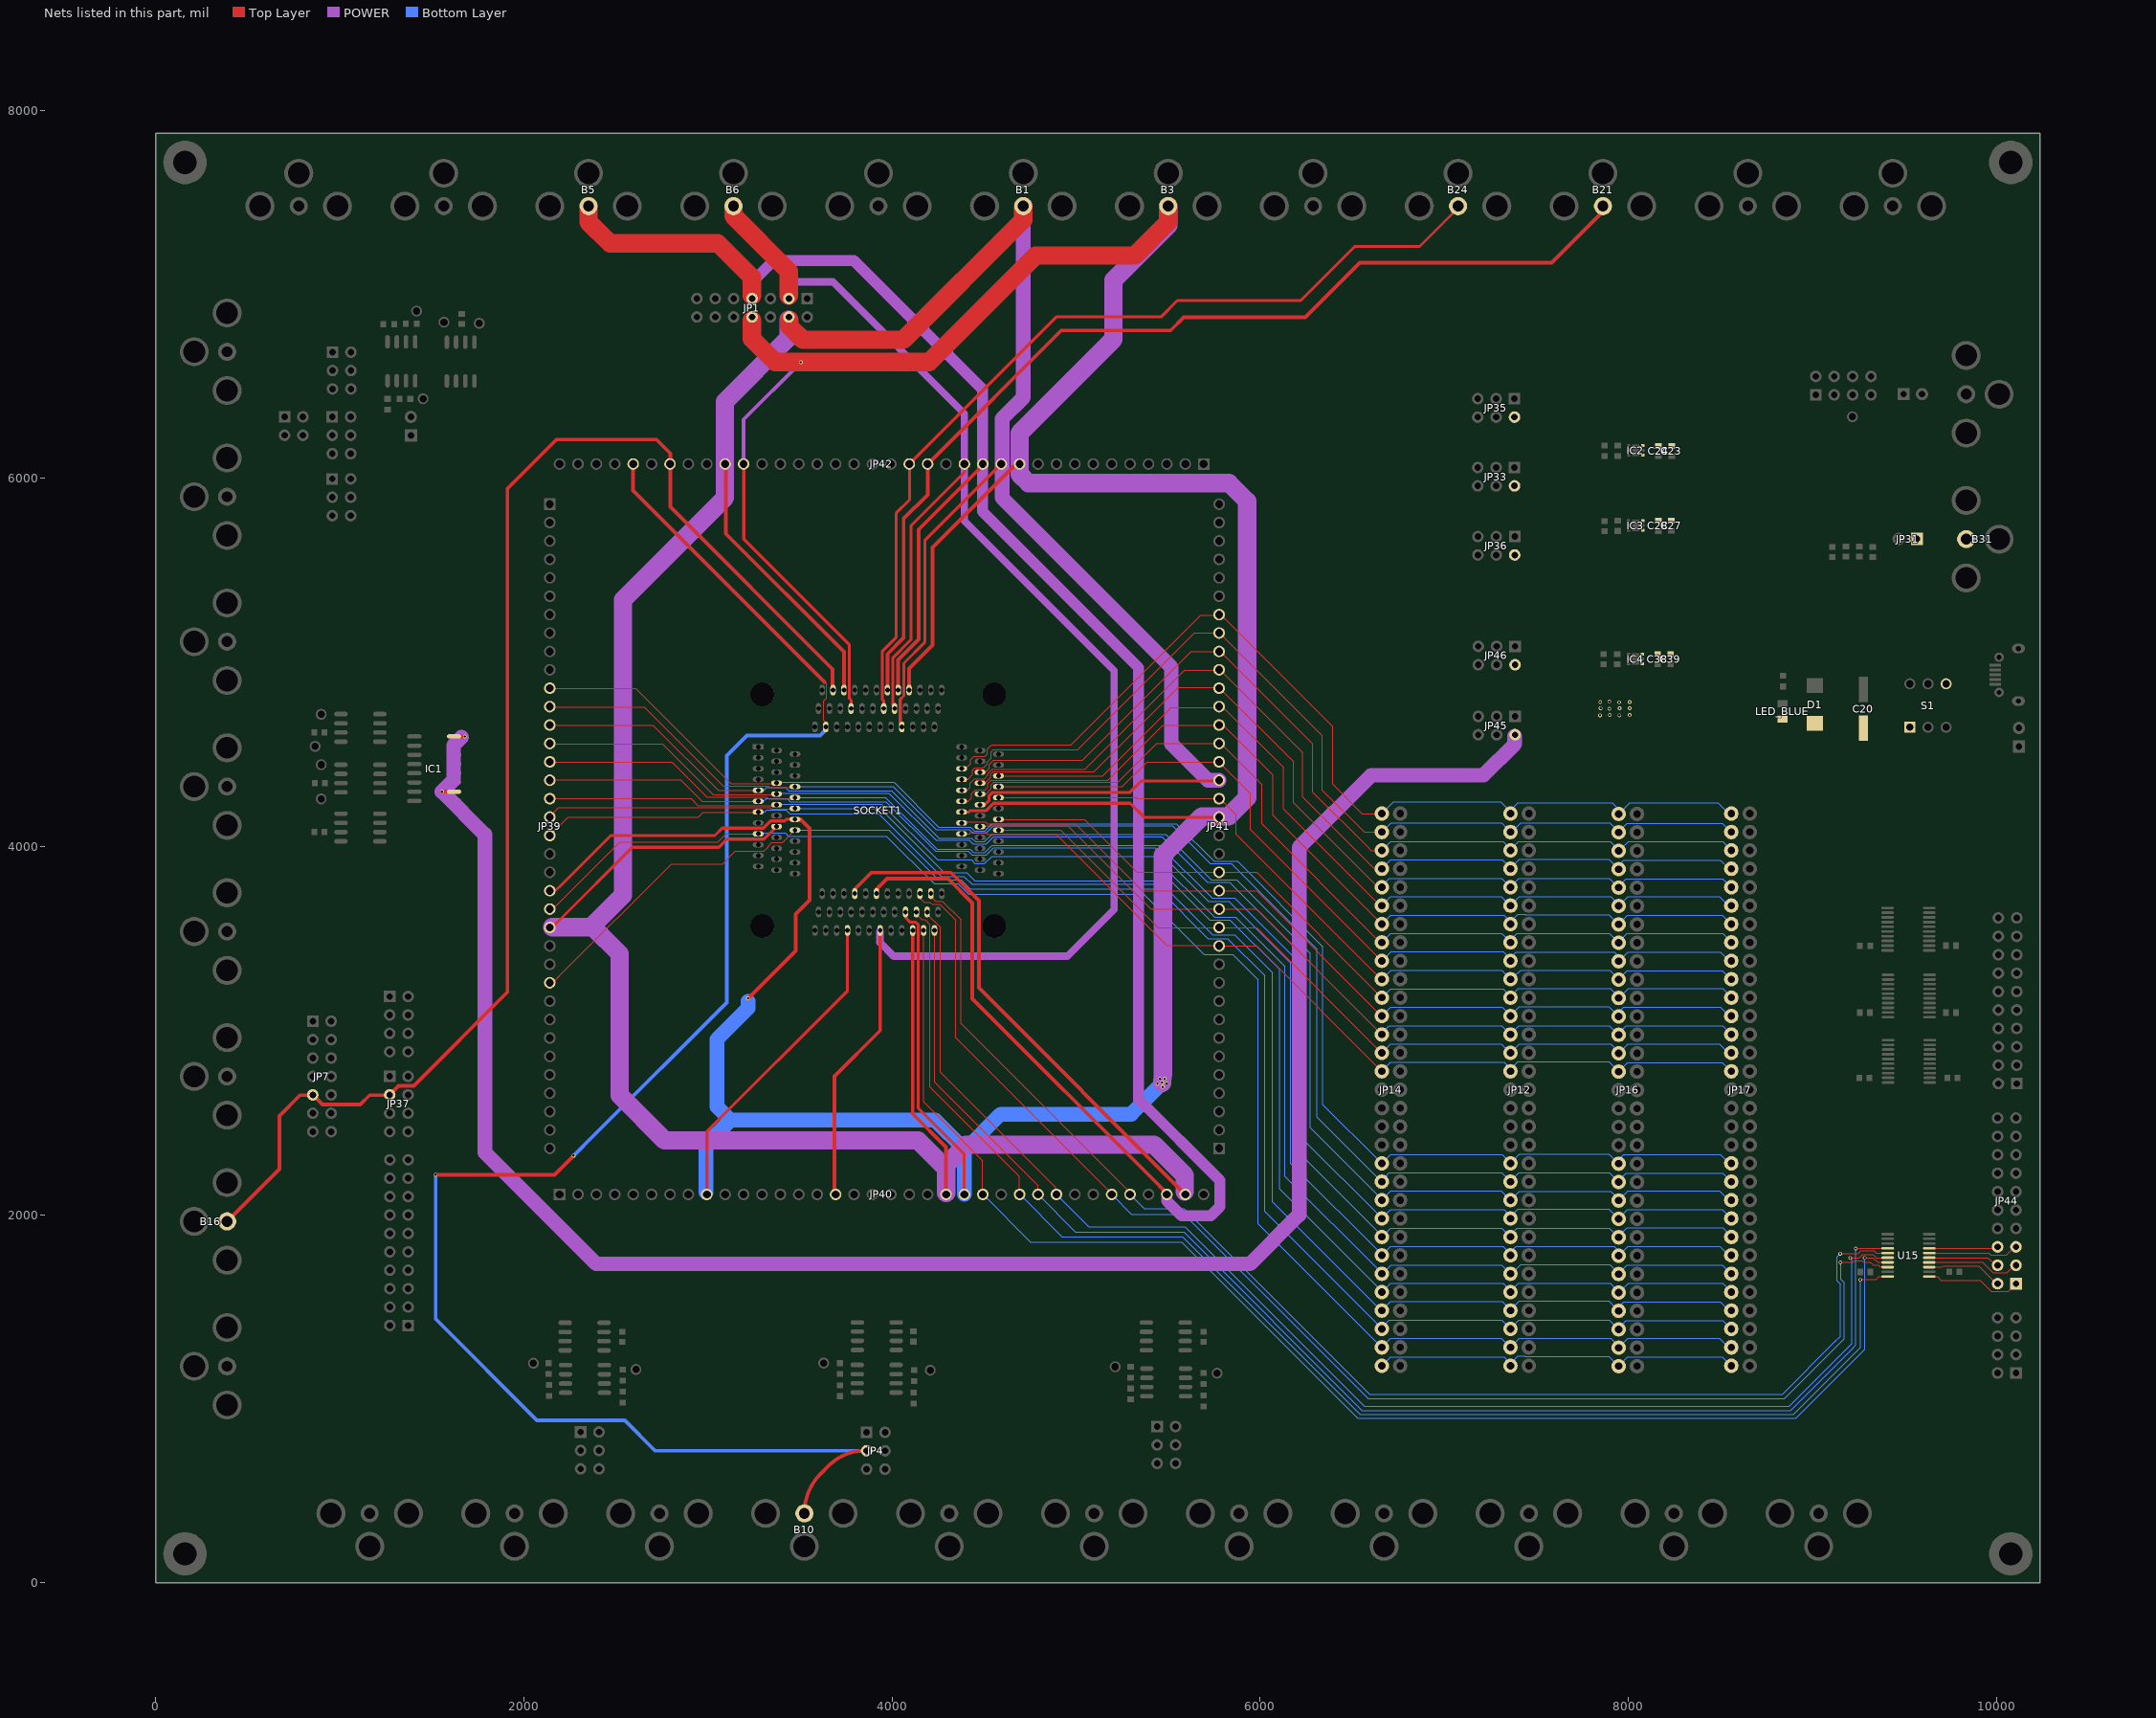
[diagram p0: the nets of this part, all layers, seen from the top]
# Altium PCB MISC62794.PcbDoc (part 5 of 7)
Units mil, origin at the board's own origin, x right, y up, seen from the top; angles counter-clockwise.
Board outline 10236.22 x 7874.02 mil, 4 copper layers (Top Layer, GND, POWER, Bottom Layer); 158 components, 185 nets, 1211 pads, 1759 vias.

## Via types
v1: diameter 20, hole 12, Top Layer to Bottom Layer, 1759 vias

## Nets (pads, with @x,y where several pads share a name; then routed paths per layer and width w, separated by ;. In a path a pad name is that pad's centre, name@x,y a point inside that pad or via, vN(x,y) a via of type N, cw(c..) or ccw(c..) an arc to the next point about the centre after c; other vN are vias at no path point) (continued)
VBIT_FORMING<4>: JP12.23 JP14.23 JP16.23 JP17.23 JP39.11 SOCKET1.11 | length 8075.9
  Top Layer w6: JP39.11@2140,4860.02 2605.98,4860.02 3125.03,4340.97 SOCKET1.11@3355.97,4340.97
  Bottom Layer w6: SOCKET1.11@3372.24,4344.65 3375.93,4348.34 4009.66,4348.34 4253.25,4104.75 4426.25,4104.75 4445.94,4085.06 4505.06,4085.06 4544.43,4124.43 5545.57,4124.43 5750.48,3919.52 5876.48,3919.52 6341,3455 6341,2598 JP14.23@6644,2295 ; JP14.23@6661,2279 6710,2328 7316,2328 7351,2293 7372,2293 7409.63,2330.63 7894.37,2330.63 7937,2288 7976,2327 8501,2327 JP17.23@8545,2283
VBIT_FORMING<5>: JP12.21 JP14.21 JP16.21 JP17.21 JP39.12 SOCKET1.12 | length 8070.4
  Top Layer w6: JP39.12@2166,4758 2654,4758 3083.03,4328.97 3327,4328.97 3334.69,4321.28 3468.56,4321.28 SOCKET1.12@3472.24,4324.97
  Bottom Layer w6: SOCKET1.12@3472.24,4324.97 4006.03,4324.97 4238.25,4092.75 4419.25,4092.75 4439,4073 4511,4073 4550.43,4112.43 5524.57,4112.43 5730,3907 5843,3907 6308,3442 6308,2530 JP14.21@6637,2201 ; JP14.21@6669,2195 6701.37,2227.37 7311.63,2227.37 JP12.21@7360,2179 ; JP12.21@7371,2192 7406.37,2227.37 7897.65,2227.37 JP16.21@7948,2177.02 ; JP16.21@7958,2196 7987.39,2225.39 8513.61,2225.39 JP17.21@8560,2179
VBIT_FORMING<6>: JP12.19 JP14.19 JP16.19 JP17.19 JP39.13 SOCKET1.13 | length 8140
  Top Layer w6: JP39.13@2140,4660.02 2700.98,4660.02 3055,4306 SOCKET1.13@3263,4306
  Bottom Layer w6: SOCKET1.13@3272.24,4305.28 3304.28,4305.28 3319,4320 3419,4320 3437.4,4301.6 3998.4,4301.6 4254.31,4045.69 4432.31,4045.69 4451.99,4026.01 4503.01,4026.01 4542.38,4065.38 5486.62,4065.38 5733,3819 5872,3819 6273,3418 6273,2472 JP14.19@6645,2100 ; JP14.19@6661,2079 6710,2128 7309,2128 JP12.19@7347,2090 ; JP12.19@7360,2079 7408.37,2127.37 7905.63,2127.37 JP16.19@7947,2086 ; JP16.19@7948,2077.02 7999.63,2128.65 8495.35,2128.65 JP17.19@8545,2079
VBIT_FORMING<7>: JP12.17 JP14.17 JP16.17 JP17.17 JP39.14 SOCKET1.14 | length 8153.6
  Top Layer w6: JP39.14@2159,4557 2752,4557 3027.09,4281.91 3368.56,4281.91 SOCKET1.14@3372.24,4285.6
  Bottom Layer w6: SOCKET1.14@3372.24,4285.6 3375.93,4289.28 3982.72,4289.28 4238.31,4033.69 4419.31,4033.69 4438.99,4014.01 4511.01,4014.01 4550.06,4053.06 5465.94,4053.06 5714,3805 5834,3805 6239,3400 6239,2402 JP14.17@6643,1998 ; JP14.17@6668,1987 6708.37,2027.37 7325.63,2027.37 7361,1992 7400,2031 7439.59,2031 7439.96,2030.63 7894.39,2030.63 JP16.17@7948,1977.02 ; JP16.17@7959,1989 7997,2027 8512,2027 JP17.17@8560,1979
VBIT_FORMING<8>: JP12.15 JP14.15 JP16.15 JP17.15 JP39.15 SOCKET1.15 | length 8237.2
  Top Layer w6: JP39.15@2140,4460.02 2803.98,4460.02 2994.09,4269.91 3320.09,4269.91 3331,4259 3462,4259 SOCKET1.15@3464,4261
  Bottom Layer w6: SOCKET1.15@3472.24,4265.91 3964.09,4265.91 4243.36,3986.64 4423.36,3986.64 4443.05,3966.95 4504.95,3966.95 4544.32,4006.32 5451.68,4006.32 5738.48,3719.52 5862.48,3719.52 6205,3377 6205,2342 JP14.15@6658,1889 ; JP14.15@6661,1879 6709.37,1927.37 7311.63,1927.37 7354,1885 7396.37,1927.37 7897.63,1927.37 7945,1880 7993.65,1928.65 8514.35,1928.65 JP17.15@8565,1878
VBIT_FORMING<9>: JP12.13 JP14.13 JP16.13 JP17.13 JP39.16 SOCKET1.16 | length 8267.5
  Top Layer w6: JP39.16@2139,4363 2851,4363 2967.77,4246.23 SOCKET1.16@3272.24,4246.23
  Bottom Layer w6: SOCKET1.16@3272.24,4246.23 3301.23,4246.23 3315,4260 3429.95,4260 3447.41,4242.54 3967.46,4242.54 4235.36,3974.64 4414.36,3974.64 4434.05,3954.95 4510.95,3954.95 4550.01,3994.01 5426.99,3994.01 5719,3702 5831,3702 6167,3366 6167,2277 JP14.13@6669,1775 ; JP14.13@6661,1779 6710,1828 7321,1828 7356,1793 7391,1828 7924,1828 7962,1790 7999,1827 8498,1827 JP17.13@8545,1780
VBIT_FORMING<10>: JP12.11 JP14.11 JP16.11 JP17.11 JP39.17 SOCKET1.17 | length 8238.2
  Top Layer w6: JP39.17@2140,4260.02 2906.98,4260.02 2944.14,4222.86 3347.86,4222.86 SOCKET1.17@3350,4225
  Bottom Layer w6: SOCKET1.17@3372.24,4226.54 3375.93,4230.23 3943.77,4230.23 4246.42,3927.58 4430.42,3927.58 4450.1,3907.9 4502.9,3907.9 4542.27,3947.27 5420.73,3947.27 5752,3616 5866,3616 6134,3348 6134,2208 JP14.11@6643,1699 ; JP14.11@6661,1679 6664.26,1679 6712.63,1727.37 7312.63,1727.37 7342,1698 7386,1698 7417,1729 7899,1729 7941,1687 7954,1687 7992.39,1725.39 8510.61,1725.39 JP17.11@8555,1681
VBIT_FORMING<11>: JP12.9 JP14.9 JP16.9 JP17.9 JP39.18 SOCKET1.18 | length 8300.9
  Top Layer w6: JP39.18@2152,4176 2186.86,4210.86 3337.14,4210.86 3344.83,4203.17 3468.56,4203.17 SOCKET1.18@3472.24,4206.86
  Bottom Layer w6: SOCKET1.18@3472.24,4206.86 3935.14,4206.86 4283,3859 4406,3859 4450,3815 5513,3815 5727.49,3600.51 5836.49,3600.51 6105,3332 6105,2140 JP14.9@6657,1588 ; JP14.9@6661,1579 6709.37,1627.37 7319.63,1627.37 7357,1590 7366,1590 7404,1628 7902,1628 7940,1590 7962,1590 8000,1628 8514,1628 JP17.9@8555,1587
VBIT_FORMING<12>: JP12.7 JP14.7 JP16.7 JP17.7 JP39.19 SOCKET1.19 | length 8380.8
  Top Layer w6: JP39.19@2140,4060.02 2240.98,4161 2947,4161 2973,4187 SOCKET1.19@3261,4187
  Bottom Layer w6: SOCKET1.19@3272.24,4187.17 3307.17,4187.17 3319,4199 3423,4199 3444,4178 3928,4178 4268,3838 4391,3838 4434,3795 5467,3795 5742.48,3519.52 5862.48,3519.52 6066,3316 6066,2070 JP14.7@6639,1497 ; JP14.7@6661,1479 6710,1528 7316,1528 7351,1493 7372,1493 7409.63,1530.63 7894.37,1530.63 7937,1488 7976,1527 8501,1527 JP17.7@8545,1483
VBIT_FORMING<13>: JP12.5 JP14.5 JP16.5 JP17.5 JP39.27 SOCKET1.24 | length 8764.5
  Top Layer w6: JP39.27@2149,3262 2158,3262 2202,3306 ; 2180,3284 2202,3306 ; SOCKET1.24@3472.24,4088.75 3404.5,4021 3346,4021 3327,4002 3327,3997.03 3304.29,3974.32 3148.32,3974.32 3080,3906 2802,3906 2202,3306
  Bottom Layer w6: SOCKET1.24@3472.24,4088.75 3883,4088.75 ; 3948.25,4088.75 3883,4088.75 ; JP14.5@6639,1404 6026,2017 6026,3298 5823.49,3500.51 5716.49,3500.51 5447,3770 4424,3770 4375,3819 4252,3819 3982.25,4088.75 3883,4088.75 ; JP14.5@6669,1395 6701.37,1427.37 7311.63,1427.37 JP12.5@7360,1379 ; JP12.5@7371,1392 7406.37,1427.37 7897.65,1427.37 JP16.5@7948,1377.02 ; JP16.5@7958,1396 7987.39,1425.39 8513.61,1425.39 JP17.5@8560,1379
VBIT_FORMING<14>: JP12.3 JP14.3 JP16.3 JP17.3 JP39.23 SOCKET1.25 | length 8606.8
  Top Layer w6: JP39.23@2149,3654 2150,3654 2521,4025 3054,4025 3098.06,4069.06 SOCKET1.25@3272.24,4069.06
  Bottom Layer w6: SOCKET1.25@3272.24,4069.06 3275.93,4072.75 SOCKET1.25@3277,4072.75 ; SOCKET1.25@3277,4069 3283,4075 3419,4075 3437,4057 3970,4057 4228,3799 4358,3799 4417,3740 5368,3740 5695,3413 5851,3413 5989,3275 5989,1951 6218,1722 JP14.3@6661,1279 6710,1328 7309,1328 JP12.3@7347,1290 ; JP12.3@7360,1279 7408.37,1327.37 7905.63,1327.37 JP16.3@7947,1286 ; JP16.3@7948,1277.02 7999.63,1328.65 8495.35,1328.65 JP17.3@8545,1279
VBIT_FORMING<15>: JP12.1 JP14.1 JP16.1 JP17.1 | length 1986.5
  Bottom Layer w6: JP14.1@6668,1187 6708.37,1227.37 7325.63,1227.37 7361,1192 7400,1231 7439.59,1231 7439.96,1230.63 7894.39,1230.63 JP16.1@7948,1177.02 ; JP16.1@7959,1189 7997,1227 8512,1227 JP17.1@8560,1179
VBIT_FORMING<16>: JP12.61 JP14.61 JP16.61 JP17.61 JP41.30 SOCKET1.102 | length 5300
  Top Layer w6: SOCKET1.102@4377.76,4423.39 4398.39,4423.39 4426,4451 4426,4473 4444,4491 4505,4491 4516.28,4502.28 4516.28,4528.28 4540,4552 4972,4552 5678,5258 JP41.30@5776,5258 ; JP41.30@5777,5260.02 5785.98,5260.02 6395,4651 6395,4338 6554,4179 JP14.61@6661,4179
  Bottom Layer w6: JP14.61@6661,4179 6724,4242 7307,4242 7356,4193 7402,4239 7913,4239 7962,4190 8009,4237 8488,4237 JP17.61@8545,4180
VBIT_FORMING<17>: JP12.57 JP14.57 JP16.57 JP17.57 JP41.28 SOCKET1.101 | length 5066.6
  Top Layer w6: SOCKET1.101@4477.76,4403.71 4507.71,4403.71 4529,4425 4529,4447 4550,4468 5034,4468 5626.02,5060.02 JP41.28@5777,5060.02 5782.98,5060.02 6286,4557 6286,4296 6584,3998 ; 6587,3995 6584,3998 ; JP14.57@6661,3979 6603,3979 6584,3998
  Bottom Layer w6: JP14.57@6661,3979 6709.37,4027.37 7319.63,4027.37 7357,3990 7366,3990 7404,4028 7902,4028 7940,3990 7962,3990 8000,4028 8514,4028 JP17.57@8555,3987
VBIT_FORMING<18>: JP12.51 JP14.51 JP16.51 JP17.51 JP41.25 SOCKET1.100 | length 4859.3
  Top Layer w6: SOCKET1.100@4577.76,4384.02 5143.02,4384.02 5515,4756 5691,4756 ; 5736.5,4756 5691,4756 ; JP41.25@5777,4760.02 5794.98,4760.02 6126,4429 6126,4204 6604,3726 ; JP41.25@5778,4758 5776,4756 5691,4756 ; 6611,3719 6604,3726 ; JP14.51@6661,3679 6651,3679 6604,3726
  Bottom Layer w6: JP14.51@6661,3679 6710,3728 7309,3728 JP12.51@7347,3690 ; JP12.51@7360,3679 7408.37,3727.37 7905.63,3727.37 JP16.51@7947,3686 ; JP16.51@7948,3677.02 7999.63,3728.65 8495.35,3728.65 JP17.51@8545,3679
VBIT_FORMING<19>: JP12.59 JP14.59 JP16.59 JP17.59 JP41.29 SOCKET1.99 | length 5265.1
  Top Layer w6: SOCKET1.99@4377.76,4364.34 4412.34,4364.34 4438,4390 4438,4415 4451,4428 4496,4428 4517,4449 4517,4452.97 4518,4453.97 4518,4460 4537,4479 4537,4514 4549,4526 5009,4526 5643.02,5160.02 JP41.29@5777,5160.02 5778.98,5160.02 6338,4601 6338,4306 6565,4079 JP14.59@6661,4079
  Bottom Layer w6: JP14.59@6661,4079 6664.26,4079 6712.63,4127.37 7312.63,4127.37 7342,4098 7386,4098 7417,4129 7899,4129 7941,4087 7954,4087 7992.39,4125.39 8510.61,4125.39 JP17.59@8555,4081
VBIT_FORMING<20>: JP12.53 JP14.53 JP16.53 JP17.53 JP41.26 SOCKET1.98 | length 4968.8
  Top Layer w6: SOCKET1.98@4477.76,4344.65 4503.65,4344.65 4535,4376 4535,4393 4549.39,4407.39 5096.39,4407.39 5554,4865 JP41.26@5777,4865 ; JP41.26@5777,4860.02 5781.98,4860.02 6181,4461 6181,4238 6600,3819 ; 6608,3811 6600,3819 ; JP14.53@6661,3779 6640,3779 6600,3819
  Bottom Layer w6: JP14.53@6669,3795 6701.37,3827.37 7311.63,3827.37 JP12.53@7360,3779 ; JP12.53@7371,3792 7406.37,3827.37 7897.65,3827.37 JP16.53@7948,3777.02 ; JP16.53@7958,3796 7987.39,3825.39 8513.61,3825.39 JP17.53@8560,3779
VBIT_FORMING<21>: JP12.45 JP14.45 JP16.45 JP17.45 JP41.22 SOCKET1.97 | length 4685.2
  Top Layer w6: SOCKET1.97@4577.76,4324.97 5250.97,4324.97 5386,4460 5395,4460 JP41.22@5777,4460.02 5777,4459 5948,4288 5948,4092 JP14.45@6661,3379
  Bottom Layer w6: JP14.45@6661,3379 6711,3429 7320,3429 7356,3393 7390.37,3427.37 7924.63,3427.37 7962,3390 7997.39,3425.39 8499.61,3425.39 JP17.45@8545,3380
VBIT_FORMING<22>: JP12.55 JP14.55 JP16.55 JP17.55 JP41.27 SOCKET1.96 | length 5187
  Top Layer w6: SOCKET1.96@4377.76,4305.28 4409.28,4305.28 4424,4320 4424,4344 4448.02,4368.02 4501.02,4368.02 4521,4388 4521,4395.97 4544.42,4419.39 5048.39,4419.39 5588,4959 5683,4959 ; 5730,4959 5683,4959 ; JP41.27@5757,4959 5683,4959 ; JP41.27@5777,4960.02 5781.98,4960.02 6232,4510 6232,4268 6597,3903 ; 6605,3895 6597,3903 ; JP14.55@6661,3879 6621,3879 6597,3903
  Bottom Layer w6: JP14.55@6661,3879 6710,3928 7316,3928 7351,3893 7372,3893 7409.63,3930.63 7894.37,3930.63 7937,3888 7976,3927 8501,3927 JP17.55@8545,3883
VBIT_FORMING<23>: JP12.47 JP14.47 JP16.47 JP17.47 JP41.23 SOCKET1.95 | length 4863.9
  Top Layer w6: SOCKET1.95@4477.76,4285.6 4508.6,4285.6 4538,4315 4538,4335 4551.34,4348.34 5226.34,4348.34 5438.02,4560.02 JP41.23@5777,4560.02 5785.98,4560.02 6009,4337 6009,4123 JP14.47@6632,3500
  Bottom Layer w6: JP14.47@6661,3479 6709.37,3527.37 7311.63,3527.37 7354,3485 7396.37,3527.37 7897.63,3527.37 7945,3480 7993.65,3528.65 8514.35,3528.65 JP17.47@8565,3478
VBIT_FORMING<24>: JP12.43 JP14.43 JP16.43 JP17.43 JP41.20 SOCKET1.94 | length 4532.7
  Top Layer w6: SOCKET1.94@4577.76,4265.91 5325.09,4265.91 ; 5325,4266 5325.09,4265.91 ; JP14.43@6651,3286 6649,3286 5870,4065 5870,4172 5781.98,4260.02 JP41.20@5777,4260.02 5330.98,4260.02 5325.09,4265.91
  Bottom Layer w6: JP14.43@6661,3279 6664.26,3279 6712.63,3327.37 7312.63,3327.37 7342,3298 7386,3298 7417,3329 7899,3329 7941,3287 7954,3287 7992.39,3325.39 8510.61,3325.39 JP17.43@8555,3281
VBIT_FORMING<25>: JP12.49 JP14.49 JP16.49 JP17.49 JP41.24 SOCKET1.93 | length 5057.6
  Top Layer w6: SOCKET1.93@4377.76,4246.23 4414.23,4246.23 4432,4264 4432,4288.05 4452.92,4308.97 4505.97,4308.97 4520,4323 4520,4343 4537.34,4360.34 5173.34,4360.34 5472,4659 5703,4659 ; 5723,4659 5703,4659 ; JP41.24@5772,4659 5703,4659 ; JP41.24@5777,4660.02 5798.98,4660.02 6070,4389 6070,4170 JP14.49@6661,3579
  Bottom Layer w6: JP14.49@6668,3587 6708.37,3627.37 7325.63,3627.37 7361,3592 7400,3631 7439.59,3631 7439.96,3630.63 7894.39,3630.63 JP16.49@7948,3577.02 ; JP16.49@7959,3589 7997,3627 8512,3627 JP17.49@8560,3579
VBIT_FORMING<26>: JP12.41 JP14.41 JP16.41 JP17.41 JP41.16 SOCKET1.88 | length 4465.3
  Top Layer w6: SOCKET1.88@4577.76,4147.8 5044.2,4147.8 5332,3860 JP41.16@5764,3860 ; JP41.16@5777,3860.02 5792,3860.02 5980,3860 JP14.41@6661,3179
  Bottom Layer w6: JP14.41@6661,3179 6709.37,3227.37 7319.63,3227.37 7357,3190 7366,3190 7404,3228 7902,3228 7940,3190 7962,3190 8000,3228 8514,3228 JP17.41@8555,3187
VBIT_FORMING<27>: JP12.39 JP14.39 JP16.39 JP17.39 JP41.15 SOCKET1.87 | length 4690.1
  Top Layer w6: SOCKET1.87@4396,4128 4401,4133 4508,4133 4516.88,4124.12 4995.88,4124.12 5359.98,3760.02 5771,3760.02 5980,3760 JP14.39@6661,3079
  Bottom Layer w6: JP14.39@6661,3079 6710,3128 7316,3128 7351,3093 7372,3093 7409.63,3130.63 7894.37,3130.63 7937,3088 7976,3127 8501,3127 JP17.39@8545,3083
VBIT_FORMING<28>: JP12.37 JP14.37 JP16.37 JP17.37 JP41.14 SOCKET1.86 | length 4615.5
  Top Layer w6: SOCKET1.86@4477.76,4108.43 4481.44,4112.12 4953.88,4112.12 5406,3660 JP41.14@5768,3660 ; JP41.14@5777,3660.02 5779,3660.02 5980,3660 JP14.37@6661,2979
  Bottom Layer w6: JP14.37@6669,2995 6701.37,3027.37 7311.63,3027.37 JP12.37@7360,2979 ; JP12.37@7371,2992 7406.37,3027.37 7897.65,3027.37 JP16.37@7948,2977.02 ; JP16.37@7958,2996 7987.39,3025.39 8513.61,3025.39 JP17.37@8560,2979
VBIT_FORMING<29>: JP12.35 JP14.35 JP16.35 JP17.35 JP41.13 SOCKET1.85 | length 4557.8
  Top Layer w6: SOCKET1.85@4592,4090 4916,4090 5445.98,3560.02 JP41.13@5777,3560.02 ; JP41.13@5775,3560 5980,3560 JP14.35@6661,2879
  Bottom Layer w6: JP14.35@6661,2879 6710,2928 7309,2928 JP12.35@7347,2890 ; JP12.35@7360,2879 7408.37,2927.37 7905.63,2927.37 JP16.35@7947,2886 ; JP16.35@7948,2877.02 7999.63,2928.65 8495.35,2928.65 JP17.35@8545,2879
VBIT_FORMING<30>: JP12.33 JP14.33 JP16.33 JP17.33 JP41.12 SOCKET1.84 | length 4805.6
  Top Layer w6: SOCKET1.84@4377.76,4069.06 4420.06,4069.06 4427,4076 4507,4076 4517.94,4065.06 4890.94,4065.06 5493,3463 JP41.12@5774,3463 ; JP41.12@5777,3460.02 5795,3460.02 5980,3460 JP14.33@6661,2779
  Bottom Layer w6: JP14.33@6668,2787 6708.37,2827.37 7325.63,2827.37 7361,2792 7400,2831 7439.59,2831 7439.96,2830.63 7894.39,2830.63 JP16.33@7948,2777.02 ; JP16.33@7959,2789 7997,2827 8512,2827 JP17.33@8560,2779
VBIT_PS_CTRL: B16.1 JP7.9 JP37.3 JP42.30 SOCKET1.139 | length 7629.6
  Top Layer w20: B16.1@386.77,1963.49 670,2246.72 670,2537 782,2649 JP7.9@835,2649 ; JP7.9@852,2651 904.5,2598.5 1110.5,2598.5 1161,2649 JP37.3@1258,2649 ; JP37.3@1269.93,2651.09 1318.83,2700 1401,2700 1910,3209 1910,5811 ; 1910,5820 1910,5811 ; SOCKET1.139@3677,4865 3677,4963 2795,5845 2795,6136 2720,6211 2176,6211 1910,5945 1910,5811
VBIT_PS_OUT1: B24.1 JP42.17 SOCKET1.125 | length 4932
  Top Layer w6: JP42.17@4093,6071 JP42.17@4093,6078.02
  Top Layer w16: SOCKET1.125@3954.53,4749.77 3954.53,4791.47 3945.84,4800.16 3945.84,5059.84 4021,5135 4021,5762 4021,5810 4095,5884 JP42.17@4095,6071 ; JP42.17@4093,6078.02 4891.98,6877 5461,6877 5550,6966 6220,6966 6514,7260 6866,7260 B24.1@7061,7455
VBIT_PS_OUT2: B21.1 JP42.16 SOCKET1.124 | length 5583.8
  Top Layer w6: SOCKET1.124@3974.21,4849.77 SOCKET1.124@3974.21,4866
  Top Layer w20: SOCKET1.124@3975,4866 3975,5046 4062,5133 4062,5780 4193,5911 JP42.16@4193,6078.02 4918.98,6804 5513,6804 5585,6876 6245,6876 6541,7172 7584,7172 B21.1@7859,7447 ; B21.1@7862.44,7447 B21.1@7862.44,7479.17
VBIT_SEL<0>: JP40.26 SOCKET1.65 U15.20 | length 7493.9
  Top Layer w6: SOCKET1.65@4131.69,3644.26 4131.69,3631.31 4160,3603 4179,3603 4206.43,3575.57 4206.43,2693.57 4692,2208 JP40.26@4692,2124 ; v1@9267,1649 9347,1649 9361.85,1663.85 U15.20@9409.97,1663.85
  Bottom Layer w6: JP40.26@4693,2110.02 4923.02,1880 5578,1880 6543,915 8898,915 9261,1278 v1(9261,1646)
VBIT_SEL<0>_MCU: JP44.1 U15.1 | length 483.8
  Top Layer w6: U15.1@9636.03,1663.85 9680.15,1663.85 9700,1644 9912,1644 9971.49,1584.51 10066.51,1584.51 JP44.1@10081,1599
VBIT_SEL<1>: JP40.31 SOCKET1.66 U15.18 | length 7376.7
  Top Layer w6: SOCKET1.66@4151.38,3744.26 4151.38,3720.62 4174,3698 4206,3698 4218,3686 4261,3686 4347,3600 4347,2960 5152,2155 ; 5162,2145 5152,2155 ; JP40.31@5183,2124 5152,2155 ; v1(9153,1741) 9221,1741 9230.5,1750.5 9271.5,1750.5 9279,1743 9315,1743 9332,1726 9359,1726 9369.97,1715.03 U15.18@9409.97,1715.03
  Bottom Layer w6: JP40.31@5193,2110.02 5300.02,2003 5587,2003 6588,1002 8849,1002 9174,1327 9174,1629 9155,1648 v1@9155,1740
VBIT_SEL<1>_MCU: JP44.2 U15.3 | length 393.5
  Top Layer w6: U15.3@9636.03,1715.03 9705.03,1715.03 9711,1721 9904,1721 JP44.2@9991,1634
VBIT_SEL<2>: JP40.24 SOCKET1.67 U15.17 | length 7737.1
  Top Layer w6: SOCKET1.67@4171.06,3544.26 4171.06,2612.94 4492,2292 4492,2262 ; JP40.24@4492,2132 4492,2262 ; 4492,2152 4492,2262 ; v1(9285,1765) 9286,1766 9330,1766 9355.38,1740.62 U15.17@9409.97,1740.62
  Bottom Layer w6: JP40.24@4493,2110.02 4751.02,1852 5573,1852 6531,894 8911,894 9285,1268 9285,1762 v1@9286,1763
VBIT_SEL<2>_MCU: JP44.3 U15.4 | length 485
  Top Layer w6: U15.4@9636.03,1740.62 9925.38,1740.62 9981.49,1684.51 10057.51,1684.51 JP44.3@10086,1713
VBIT_SEL<3>: JP40.28 SOCKET1.68 U15.16 | length 7484.5
  Top Layer w6: SOCKET1.68@4190.75,3644.26 4190.75,3631.84 4262,3560.59 4262,2774 4848,2188 ; 4882,2154 4848,2188 ; JP40.28@4889,2119 4889,2147 4848,2188 ; v1@9213,1766 9254,1766 9272,1784 9331,1784 9348.78,1766.22 U15.16@9409.97,1766.22
  Bottom Layer w6: JP40.28@4893,2110.02 5069.02,1934 5591,1934 6567,958 8874,958 9215,1299 9215,1756 v1(9206,1765)
VBIT_SEL<3>_MCU: JP44.4 U15.5 | length 372.8
  Top Layer w6: U15.5@9636.03,1766.22 9954.78,1766.22 JP44.4@9993,1728
VBIT_SEL<4>: JP40.32 SOCKET1.69 U15.15 | length 7307.9
  Top Layer w6: SOCKET1.69@4210.43,3744.26 4210.43,3729.57 4237,3703 4274,3703 4374,3603 4374,3040 5240,2174 ; 5267,2147 5240,2174 ; JP40.32@5292,2122 5240,2174 ; v1@9158,1789 9250,1789 9265,1804 9336,1804 9348.19,1791.81 U15.15@9409.97,1791.81
  Bottom Layer w6: JP40.32@5293,2110.02 5370.02,2033 5586,2033 6594,1025 8838,1025 9120.5,1307.5 ; 9128.5,1315.5 9120.5,1307.5 ; v1(9152,1788) 9134,1770 9134,1640 9153,1621 9153,1340 9120.5,1307.5
VBIT_SEL<4>_MCU: JP44.5 U15.6 | length 468.1
  Top Layer w6: U15.6@9636.03,1791.81 9958.19,1791.81 9970,1780 10054,1780 JP44.5@10086,1812
VBIT_SEL<5>: JP40.27 SOCKET1.70 U15.14 | length 7442.1
  Top Layer w6: SOCKET1.70@4230.12,3544.26 4230.12,2719.88 4792,2158 JP40.27@4792,2116 ; v1@9238.6,1817.4 U15.14@9409.97,1817.4
  Bottom Layer w6: JP40.27@4793,2110.02 4997.02,1906 5585,1906 6554,937 8882,937 9217,1272 ; 9223.5,1278.5 9217,1272 ; v1(9236,1816) 9236,1291 9217,1272
VBIT_SEL<5>_MCU: JP44.6 U15.7 | length 354.4
  Top Layer w6: U15.7@9636.03,1817.4 JP44.6@9990.4,1817.4
VCC_5V: B31.1 C20.1 C23.1 C24.1 C27.1 C28.1 C38.1 C39.1 D1.1 IC1.10 IC1.16 IC2.4 IC2.6 IC3.4 IC3.6 IC4.4 IC4.6 JP31.1 JP33.2 JP35.2 JP36.2 JP45.2 JP46.2 LED_BLUE.1 S1.1 S1.6 | length 10749.2
  Top Layer w20: v1(1554.08,4298.08) IC1.10@1619.33,4298.08 ; IC1.16@1619.33,4598.08 v1(1677.92,4598.08)
  POWER w80: 1661,4594 1617,4550 1617,4361 v1(1554.08,4298.08) 1787,4065.16 1787,2338 2392,1733 5945,1733 6212,2000 6212,3996 6603,4387 7213,4387 7383,4557 JP45.2@7383,4600
  other v1: 7847,4713 7952,4713 8008,4714 7900,4715 7897,4749 7953,4751 8008,4751 7850,4752 7951,4784 7848,4785 8008,4785 7897,4787
VDD: B6.1 JP1.3 JP40.16 JP42.14 SOCKET1.55 SOCKET1.122 | length 9463.5
  Top Layer w16: SOCKET1.122@4015,4758 4004.9,4768.1 4004.9,5025.9 4102,5123 4102,5742 4393,6033 JP42.14@4393,6078.02
  Top Layer w20: JP40.16@3687,2124 3687,2185 ; 3687,2171 3687,2185 ; SOCKET1.55@3934.84,3544.26 3934.84,2999.84 3687,2752 3687,2185
  Top Layer w40: JP1.3@3439,6977 JP1.3@3439,6994
  Top Layer w100: B6.1@3138.03,7479.17 3138.03,7425.97 3439,7125 JP1.3@3439,6994
  POWER w40: JP1.3@3439,6977 3439,7024 3483,7068 3677,7068 4393,6352 JP42.14@4393,6078.02 4393,5769 5206,4956 5206,3658 4952,3404 4009,3404 3934,3479 SOCKET1.55@3934,3539
VDD25: B5.1 JP1.7 JP40.34 JP42.13 SOCKET1.54 SOCKET1.121 | length 12283.8
  Top Layer w20: SOCKET1.54@3915.16,3744.26 3915.16,3768.16 3973,3826 4304,3826 4436,3694 4436,3173 5443.5,2165.5 ; SOCKET1.121@4033.27,4849.77 4033.27,5014.27 4144,5125 4144,5722 JP42.13@4482,6060 ; 5460,2149 5443.5,2165.5 ; JP40.34@5492,2117 5443.5,2165.5
  Top Layer w100: B5.1@2350.63,7479.17 2350.63,7393.37 2467,7277 3053,7277 3238,7092 JP1.7@3238,6994
  POWER w60: JP1.7@3239,6977 3239,7065 3357,7183 3544,7183 3792,7183 4491,6484 4491,5820 5340,4971 5340,2627 5781,2186 5781,2044 5731,1994 5573,1994 5493,2074 JP40.34@5493,2110.02
VDDC: B3.1 JP1.8 JP39.22 JP40.9 JP40.23 JP41.19 JP42.11 JP42.26 SOCKET1.21 SOCKET1.46 SOCKET1.62 SOCKET1.90 SOCKET1.118 SOCKET1.134 | length 24695.1
  Top Layer w16: JP39.22@2149,3763 2174,3763 2204.5,3793.5 ; 2192,3781 2204.5,3793.5 ; JP40.9@2994,2121 2994,2192 ; 2994,2156 2994,2192 ; JP42.26@3194,6065 3194,5671 3766.36,5098.64 3766.36,4806.64 3777.36,4795.64 SOCKET1.134@3777.36,4749.77 ; SOCKET1.21@3472.24,4147.8 3423.8,4147.8 3415,4139 3340,4139 3300.75,4099.75 3076.75,4099.75 3037,4060 2471,4060 2204.5,3793.5 ; SOCKET1.46@3757.68,3544.26 3757.68,3216.68 2994,2453 2994,2192 ; SOCKET1.62@4074,3625 4074,3613 4099,3588 4128.9,3588 4142.69,3574.2 4142.69,2577.31 4392,2328 4392,2246 ; SOCKET1.90@4377.76,4187.17 4416.17,4187.17 4424.86,4195.86 4511.48,4195.86 4550.85,4235.23 5293.77,4235.23 5370,4159 5669,4159 ; JP40.23@4392,2117 4392,2246 ; 4392,2202 4392,2246 ; 5716,4159 5669,4159 ; JP41.19@5764,4159 5669,4159
  Top Layer w20: v1(3217,3176) 3218,3176 3476,3434 3476,3634 3551,3709 3551,4099 3502.2,4147.8 SOCKET1.21@3472.24,4147.8 ; SOCKET1.118@4092.32,4849.77 4092.32,4966.32 4220,5094 4220,5625 JP42.11@4678,6083
  Top Layer w80: JP1.8@3239,6860 JP1.8@3239,6869
  Top Layer w100: JP1.8@3238,6860 3238,6759 3365,6632 4201,6632 4780,7211 5319,7211 5500.24,7392.24 B3.1@5500.24,7479.17
  POWER w20: JP42.26@3193,6078.02 3193,6320 v1(3504,6631)
  POWER w80: B3.1@5500.24,7467 B3.1@5500.24,7479.17
  POWER w100: v1@5467,2716 5470,2757 ; 5471,2762 5471,3952 5683,4164 5828,4164 5929,4265 5929,5876 5830,5975 4741,5975 4693,6023 JP42.11@4693,6078.02 4693,6246 5203,6756 5203,7077 5500.24,7374.24 B3.1@5500.24,7479.17
  Bottom Layer w80: JP40.9@2988,2121 2988,2379 3122,2513 ; 3217,3160 3217,3121 3048,2952 3048,2587 3122,2513 ; JP40.23@4393,2110.02 4393,2349 4590,2546 5299,2546 v1@5471,2718 ; 4393,2354 4234,2513 3122,2513
  other v1: 5470,2694 5442,2711 5492,2712 5467,2718 5456,2738 5481,2738
VDDH: B1.1 JP1.4 JP39.24 JP40.22 JP40.35 JP41.21 JP42.12 JP42.27 SOCKET1.23 SOCKET1.48 SOCKET1.64 SOCKET1.92 SOCKET1.120 SOCKET1.136 | length 24281.4
  Top Layer w16: JP39.24@2145,3560 2152,3560 2189,3597 ; 2181,3589 2189,3597 ; SOCKET1.23@3372.24,4108.43 3303.81,4040 3102,4040 3058,3996 2588,3996 2189,3597 ; SOCKET1.120@4054,4659 4044.27,4668.73 4044.27,4799.27 4063.95,4818.95 4063.95,4995.95 4177,5109 4177,5662.02 JP42.12@4593,6078.02 ; SOCKET1.92@4477.76,4226.54 4503.54,4226.54 4527,4250 4527,4276 4545.28,4294.28 5292.28,4294.28 5353,4355 5687,4355 ; 5710,4355 5687,4355 ; JP41.21@5767,4355 5687,4355
  Top Layer w20: JP42.27@3097,6073 3097,5699 3738,5058 SOCKET1.136@3738,4869 ; SOCKET1.48@3797.05,3744.26 3797.05,3769.05 3886,3858 4320,3858 4471,3707 4471,3232.02 JP40.35@5593,2110.02 ; SOCKET1.64@4112.01,3544.26 4112.01,2547.99 4293,2367 JP40.22@4293,2110.02
  Top Layer w80: JP1.4@3439,6868 3439,6834 3441,6832
  Top Layer w100: JP1.4@3441,6860 3441,6832 3441,6827 3515,6753 4061,6753 4712.84,7404.84 B1.1@4712.84,7479.17
  POWER w80: JP40.22@4293,2110.02 JP40.22@4293,2119 ; B1.1@4712.84,7479.17 4712.84,6439.84 4597,6324 4597,5896 4946,5547 4946,5546 5517,4975 5517,4558 5714.98,4360.02 JP41.21@5777,4360.02 ; JP40.35@5585,2117 JP40.35@5585,2125
  POWER w100: JP39.24@2153,3562 2363,3562 2537,3736 2537,5340 3092,5895 3092,6418 3439,6765 JP1.4@3439,6863 ; 2374,3562 2520,3416 2520,2648 2764,2404 4140,2404 4293.5,2250.5 ; JP40.22@4294,2119 4294,2271 4403,2380 5424,2380 5590,2214 JP40.35@5590,2125
VG1: B10.1 JP4.3 JP42.32 SOCKET1.141 | length 9742.1
  Top Layer w6: 3632.5,4894.5 3643.25,4883.75 3643.25,4806.25 3629,4792 3629,4685 3639.57,4674.43 SOCKET1.141@3639.57,4649.77
  Top Layer w20: v1(1520,2217) 2165,2217 v1(2269,2321) ; JP42.32@2593,6078.02 2593,5934.76 3632.88,4894.88 ; B10.1@3523.2,377.15 cw(c3829.94,377.15) 3613.04,594.04 3653.15,634.15 cw(c3858,429.29) JP4.3@3858,719
  Bottom Layer w20: v1(1520,2217) 1520,1433 2070,883 2547,883 2712.62,717.38 JP4.3@3861.48,717.38 ; v1(2269,2321) 2383,2435 3101,3153 3101,4493 3211,4603 3609,4603 3639.57,4633.57 SOCKET1.141@3639.57,4649.77